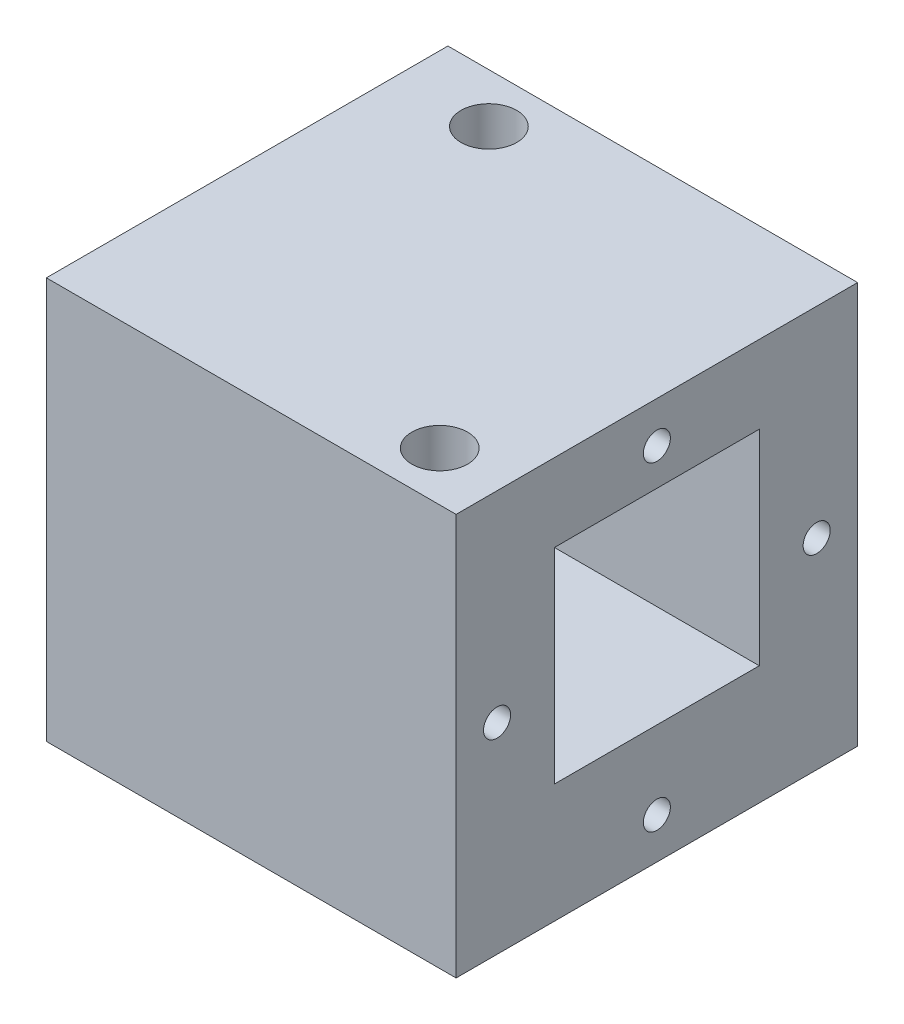
SolidWorks part; units mm, degrees
ref_plane "前视基准面" through (0, 0, 0) normal (0, 0, 1) x (1, 0, 0)
ref_plane "上视基准面" through (0, 0, 0) normal (0, 1, 0) x (1, 0, 0)
ref_plane "右视基准面" through (0, 0, 0) normal (1, 0, 0) x (0, 0, -1)
sketch "草图2" plane through (0, 0, 0) normal (1, 0, 0) x (0, 0, -1)
  line L1 (0, 0) -> (49, 0)
  line L2 (0, 0) -> (0, 49)
  line L3 (0, 49) -> (49, 49)
  line L4 (49, 0) -> (49, 49)
  dimension "D1" = 49
  dimension "D2" = 49
extrude "凸台-拉伸2" add sketch "草图2" along normal blind 50
sketch "草图3" plane through (50, 0, 0) normal (1, 0, 0) x (0, 0, -1)
  line L0 (24.5, 0) -> (24.5, 62.022) construction
  line L1 (12, 39.5) -> (37, 39.5)
  line L2 (12, 39.5) -> (12, 14.5)
  line L3 (12, 14.5) -> (37, 14.5)
  line L4 (37, 39.5) -> (37, 14.5)
  line L5 (0, 0) -> (49, 0) construction
  line L6 (0, 24.5) -> (65.441, 24.5) construction
  line L7 (0, 49) -> (0, 0) construction
  dimension "D1" = 25
  dimension "D2" = 25
  dimension "D3" = 12.5
  dimension "D4" = 15
extrude "切除-拉伸1" cut sketch "草图3" against normal blind 50
hole_wizard "M4 螺纹孔1" positions "草图5" profile "草图4" tap size "M4" standard "GB"
sketch "草图5" plane through (50, 0, 0) normal (1, 0, 0) x (0, 0, -1)
  line L1 (24.5, 49) -> (24.5, -5.0027) construction
  line L2 (49, 49) -> (0, 49) construction
  line L4 (0, 24.5) -> (58.6427, 24.5) construction
  line L5 (0, 49) -> (0, 0) construction
  line L7 (0, 0) -> (49, 0) construction
  line L8 (49, 0) -> (49, 49) construction
  point P0 (24.5, 44)
  point P1 (5, 24.5)
  point P3 (24.5, 5)
  point P5 (44, 24.5)
  dimension "D1" = 5
  dimension "D2" = 5
  dimension "D3" = 5
  dimension "D4" = 5
sketch "草图4" plane through (50, 44, -24.5) normal (0, 1, 0) x (0, 0, -1)
  line L0 (0, 0) -> (0, 14.4914)
  line L1 (0, 14.4914) -> (1.65, 13.5)
  line L2 (1.65, 13.5) -> (1.65, 0)
  line L5 (1.65, 0) -> (0, 0)
  line L10 (0, 14.4914) -> (-1.65, 13.5) construction
  line L11 (0, -6.35) -> (0, 107.95) construction
  dimension "螺纹孔钻头直径" = 3.3
  dimension "螺纹孔钻头深度" = 13.5
  dimension "导头角度" = 118
cosmetic thread "孔螺蚊线1" parameters "D1"=10, "D2"=4
cosmetic thread "孔螺蚊线2" parameters "D1"=10, "D2"=4
cosmetic thread "孔螺蚊线3" parameters "D1"=10, "D2"=4
cosmetic thread "孔螺蚊线4" parameters "D1"=10, "D2"=4
hole_wizard "M8 螺纹孔1" positions "草图7" profile "草图6" tap size "M8" standard "GB"
sketch "草图7" plane through (0, 49, 0) normal (0, 1, 0) x (-1, 0, 0)
  line L0 (0, -49) -> (0, 0) construction
  line L2 (0, -24.5) -> (-61.8244, -24.5) construction
  point P0 (-42, -6)
  point P1 (-11, -43)
  dimension "D1" = 42
  dimension "D2" = 11
  dimension "D3" = 18.5
  dimension "D4" = 18.5
sketch "草图6" plane through (42, 49, -6) normal (1, 0, 0) x (0, 0, 1)
  line L0 (0, 0) -> (0, 20.0429)
  line L1 (0, 20.0429) -> (3.4, 18)
  line L2 (3.4, 18) -> (3.4, 0)
  line L5 (3.4, 0) -> (0, 0)
  line L10 (0, 20.0429) -> (-3.4, 18) construction
  line L11 (0, -6.35) -> (0, 107.95) construction
  dimension "螺纹孔钻头直径" = 6.8
  dimension "螺纹孔钻头深度" = 18
  dimension "导头角度" = 118
cosmetic thread "孔螺蚊线5" parameters "D1"=16, "D2"=8
cosmetic thread "孔螺蚊线6" parameters "D1"=16, "D2"=8
